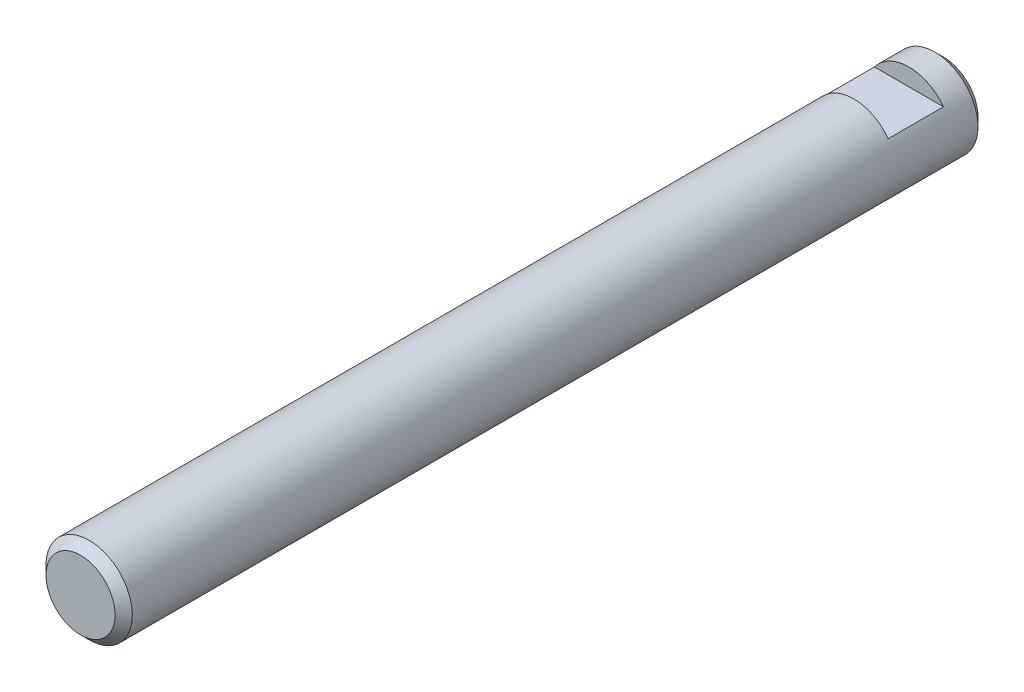
from build123d import *

# Parameters (mm, degrees)
SKETCH_1_R               = 2.5
EXTRUDE_1_DEPTH          = 25
CHAMFER_1_SIZE           = 0.5
CUT_EXTRUDE_1_DEPTH      = 26.248762346
CUT_EXTRUDE_1_DEPTH_BACK = 26.248762346
SKETCH_2_W               = 3.2
SKETCH_2_H               = 3.525136196


with BuildPart() as part:
    # 草图1 → 凸台-拉伸1 (new, symmetric)
    with BuildSketch(Plane.XY):
        Circle(SKETCH_1_R)
    extrude(amount=EXTRUDE_1_DEPTH, both=True)

    # 倒角1
    chamfer_1_edges = [part.edges().sort_by_distance(p)[0] for p in [
        (-2.5, 0, -25),
        (-2.5, 0, 25),
    ]]
    chamfer(chamfer_1_edges, length=CHAMFER_1_SIZE)

    # 草图2 → 切除-拉伸1 (cut, two sides: drawn at the far end of the back side and taken through both)
    with BuildSketch(Plane(origin=(0, 0, 0), x_dir=(0, 0, -1), z_dir=(1, 0, 0)).offset(-CUT_EXTRUDE_1_DEPTH_BACK)):
        with Locations((21.4, 3.262568098)):
            Rectangle(SKETCH_2_W, SKETCH_2_H)
    extrude(amount=CUT_EXTRUDE_1_DEPTH + CUT_EXTRUDE_1_DEPTH_BACK, mode=Mode.SUBTRACT)


solid = part.part
